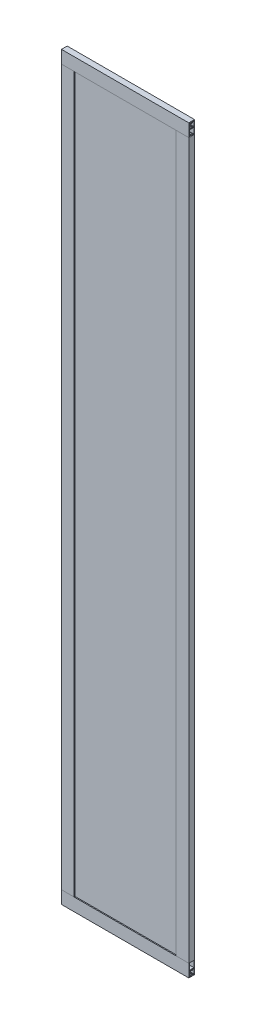
from build123d import *

# Parameters (mm, degrees)
MEMBER_1_DEPTH   = 398.5
MEMBER_1_2_DEPTH = 398.5
MEMBER_1_3_DEPTH = 2319
MEMBER_1_4_DEPTH = 2319
EXTRUDE_START    = -3.1
SKETCH_2_W       = 352.5
SKETCH_2_H       = 2271
EXTRUDE_1_DEPTH  = 10


with BuildPart() as part:
    # Sketch1 → Member 1 (new body)
    with BuildSketch(Plane(origin=(-199.25, 1158.5, 0), x_dir=(0, 0, -1), z_dir=(1, 0, 0))):
        Polygon((7, -38.5), (5.9, -38.5), (5.9, -40), (7, -40), (9, -40), (9, 0), (-9, 0), (-9, -40), (-7, -40), (-5.9, -40), (-5.9, -38.5), (-7, -38.5), (-7, -20), (7, -20), align=None)
        with BuildLine():
            Line((-1.341640786, -18), (1.341640786, -18))
            ThreePointArc((1.341640786, -18), (1.799302724, -16.749903013), (1.272792206, -15.527207794))
            ThreePointArc((1.272792206, -15.527207794), (1.272792206, -14.749390335), (2.050609665, -14.749390335))
            ThreePointArc((2.050609665, -14.749390335), (2.853462499, -16.282552641), (2.640075756, -18))
            Line((2.640075756, -18), (7, -18))
            Line((7, -18), (7, -3))
            Line((7, -3), (2.640075756, -3))
            ThreePointArc((2.640075756, -3), (2.853462499, -4.717447359), (2.050609665, -6.250609665))
            ThreePointArc((2.050609665, -6.250609665), (1.272792206, -6.250609665), (1.272792206, -5.472792206))
            ThreePointArc((1.272792206, -5.472792206), (1.799302724, -4.250096987), (1.341640786, -3))
            Line((1.341640786, -3), (-1.341640786, -3))
            ThreePointArc((-1.341640786, -3), (-1.799302724, -4.250096987), (-1.272792206, -5.472792206))
            ThreePointArc((-1.272792206, -5.472792206), (-1.272792206, -6.250609665), (-2.050609665, -6.250609665))
            ThreePointArc((-2.050609665, -6.250609665), (-2.853462499, -4.717447359), (-2.640075756, -3))
            Line((-2.640075756, -3), (-7, -3))
            Line((-7, -3), (-7, -18))
            Line((-7, -18), (-2.640075756, -18))
            ThreePointArc((-2.640075756, -18), (-2.853462499, -16.282552641), (-2.050609665, -14.749390335))
            ThreePointArc((-2.050609665, -14.749390335), (-1.272792206, -14.749390335), (-1.272792206, -15.527207794))
            ThreePointArc((-1.272792206, -15.527207794), (-1.799302724, -16.749903013), (-1.341640786, -18))
        make_face(mode=Mode.SUBTRACT)
    extrude(amount=MEMBER_1_DEPTH)


with BuildPart() as body_2:
    # Sketch1 on segment 2 (carried to segment 2) → Member 1 2 (new body)
    with BuildSketch(Plane(origin=(-199.25, -1158.5, 0), x_dir=(0, 0, 1), z_dir=(1, 0, 0))):
        Polygon((7, -38.5), (5.9, -38.5), (5.9, -40), (7, -40), (9, -40), (9, 0), (-9, 0), (-9, -40), (-7, -40), (-5.9, -40), (-5.9, -38.5), (-7, -38.5), (-7, -20), (7, -20), align=None)
        with BuildLine():
            Line((-1.341640786, -18), (1.341640786, -18))
            ThreePointArc((1.341640786, -18), (1.799302724, -16.749903013), (1.272792206, -15.527207794))
            ThreePointArc((1.272792206, -15.527207794), (1.272792206, -14.749390335), (2.050609665, -14.749390335))
            ThreePointArc((2.050609665, -14.749390335), (2.853462499, -16.282552641), (2.640075756, -18))
            Line((2.640075756, -18), (7, -18))
            Line((7, -18), (7, -3))
            Line((7, -3), (2.640075756, -3))
            ThreePointArc((2.640075756, -3), (2.853462499, -4.717447359), (2.050609665, -6.250609665))
            ThreePointArc((2.050609665, -6.250609665), (1.272792206, -6.250609665), (1.272792206, -5.472792206))
            ThreePointArc((1.272792206, -5.472792206), (1.799302724, -4.250096987), (1.341640786, -3))
            Line((1.341640786, -3), (-1.341640786, -3))
            ThreePointArc((-1.341640786, -3), (-1.799302724, -4.250096987), (-1.272792206, -5.472792206))
            ThreePointArc((-1.272792206, -5.472792206), (-1.272792206, -6.250609665), (-2.050609665, -6.250609665))
            ThreePointArc((-2.050609665, -6.250609665), (-2.853462499, -4.717447359), (-2.640075756, -3))
            Line((-2.640075756, -3), (-7, -3))
            Line((-7, -3), (-7, -18))
            Line((-7, -18), (-2.640075756, -18))
            ThreePointArc((-2.640075756, -18), (-2.853462499, -16.282552641), (-2.050609665, -14.749390335))
            ThreePointArc((-2.050609665, -14.749390335), (-1.272792206, -14.749390335), (-1.272792206, -15.527207794))
            ThreePointArc((-1.272792206, -15.527207794), (-1.799302724, -16.749903013), (-1.341640786, -18))
        make_face(mode=Mode.SUBTRACT)
    extrude(amount=MEMBER_1_2_DEPTH)


with BuildPart() as body_3:
    # Sketch1 on segment 3 (carried to segment 3) → Member 1 3 (new body)
    with BuildSketch(Plane(origin=(-199.25, 1159.5, 0), x_dir=(0, 0, 1), z_dir=(0, -1, 0))):
        Polygon((7, -38.5), (5.9, -38.5), (5.9, -40), (7, -40), (9, -40), (9, 0), (-9, 0), (-9, -40), (-7, -40), (-5.9, -40), (-5.9, -38.5), (-7, -38.5), (-7, -20), (7, -20), align=None)
        with BuildLine():
            Line((-1.341640786, -18), (1.341640786, -18))
            ThreePointArc((1.341640786, -18), (1.799302724, -16.749903013), (1.272792206, -15.527207794))
            ThreePointArc((1.272792206, -15.527207794), (1.272792206, -14.749390335), (2.050609665, -14.749390335))
            ThreePointArc((2.050609665, -14.749390335), (2.853462499, -16.282552641), (2.640075756, -18))
            Line((2.640075756, -18), (7, -18))
            Line((7, -18), (7, -3))
            Line((7, -3), (2.640075756, -3))
            ThreePointArc((2.640075756, -3), (2.853462499, -4.717447359), (2.050609665, -6.250609665))
            ThreePointArc((2.050609665, -6.250609665), (1.272792206, -6.250609665), (1.272792206, -5.472792206))
            ThreePointArc((1.272792206, -5.472792206), (1.799302724, -4.250096987), (1.341640786, -3))
            Line((1.341640786, -3), (-1.341640786, -3))
            ThreePointArc((-1.341640786, -3), (-1.799302724, -4.250096987), (-1.272792206, -5.472792206))
            ThreePointArc((-1.272792206, -5.472792206), (-1.272792206, -6.250609665), (-2.050609665, -6.250609665))
            ThreePointArc((-2.050609665, -6.250609665), (-2.853462499, -4.717447359), (-2.640075756, -3))
            Line((-2.640075756, -3), (-7, -3))
            Line((-7, -3), (-7, -18))
            Line((-7, -18), (-2.640075756, -18))
            ThreePointArc((-2.640075756, -18), (-2.853462499, -16.282552641), (-2.050609665, -14.749390335))
            ThreePointArc((-2.050609665, -14.749390335), (-1.272792206, -14.749390335), (-1.272792206, -15.527207794))
            ThreePointArc((-1.272792206, -15.527207794), (-1.799302724, -16.749903013), (-1.341640786, -18))
        make_face(mode=Mode.SUBTRACT)
    extrude(amount=MEMBER_1_3_DEPTH)

    # Member 1 3 end butt 1
    split(bisect_by=Plane(origin=(-199.25, 1118.5, 0), x_dir=(1, 0, 0), z_dir=(0, -1, 0)), keep=Keep.TOP)

    # Member 1 3 end butt 2
    split(bisect_by=Plane(origin=(-199.25, -1118.5, 0), x_dir=(-1, 0, 0), z_dir=(0, 1, 0)), keep=Keep.TOP)


with BuildPart() as body_4:
    # Sketch1 on segment 4 (carried to segment 4) → Member 1 4 (new body)
    with BuildSketch(Plane(origin=(199.25, 1159.5, 0), x_dir=(0, 0, -1), z_dir=(0, -1, 0))):
        Polygon((7, -38.5), (5.9, -38.5), (5.9, -40), (7, -40), (9, -40), (9, 0), (-9, 0), (-9, -40), (-7, -40), (-5.9, -40), (-5.9, -38.5), (-7, -38.5), (-7, -20), (7, -20), align=None)
        with BuildLine():
            Line((-1.341640786, -18), (1.341640786, -18))
            ThreePointArc((1.341640786, -18), (1.799302724, -16.749903013), (1.272792206, -15.527207794))
            ThreePointArc((1.272792206, -15.527207794), (1.272792206, -14.749390335), (2.050609665, -14.749390335))
            ThreePointArc((2.050609665, -14.749390335), (2.853462499, -16.282552641), (2.640075756, -18))
            Line((2.640075756, -18), (7, -18))
            Line((7, -18), (7, -3))
            Line((7, -3), (2.640075756, -3))
            ThreePointArc((2.640075756, -3), (2.853462499, -4.717447359), (2.050609665, -6.250609665))
            ThreePointArc((2.050609665, -6.250609665), (1.272792206, -6.250609665), (1.272792206, -5.472792206))
            ThreePointArc((1.272792206, -5.472792206), (1.799302724, -4.250096987), (1.341640786, -3))
            Line((1.341640786, -3), (-1.341640786, -3))
            ThreePointArc((-1.341640786, -3), (-1.799302724, -4.250096987), (-1.272792206, -5.472792206))
            ThreePointArc((-1.272792206, -5.472792206), (-1.272792206, -6.250609665), (-2.050609665, -6.250609665))
            ThreePointArc((-2.050609665, -6.250609665), (-2.853462499, -4.717447359), (-2.640075756, -3))
            Line((-2.640075756, -3), (-7, -3))
            Line((-7, -3), (-7, -18))
            Line((-7, -18), (-2.640075756, -18))
            ThreePointArc((-2.640075756, -18), (-2.853462499, -16.282552641), (-2.050609665, -14.749390335))
            ThreePointArc((-2.050609665, -14.749390335), (-1.272792206, -14.749390335), (-1.272792206, -15.527207794))
            ThreePointArc((-1.272792206, -15.527207794), (-1.799302724, -16.749903013), (-1.341640786, -18))
        make_face(mode=Mode.SUBTRACT)
    extrude(amount=MEMBER_1_4_DEPTH)

    # Member 1 4 end butt 1
    split(bisect_by=Plane(origin=(199.25, 1118.5, 0), x_dir=(1, 0, 0), z_dir=(0, -1, 0)), keep=Keep.TOP)

    # Member 1 4 end butt 2
    split(bisect_by=Plane(origin=(199.25, -1118.5, 0), x_dir=(-1, 0, 0), z_dir=(0, 1, 0)), keep=Keep.TOP)


with BuildPart() as body_5:
    # 草图2 → 凸台-拉伸1 (new body)
    with BuildSketch(Plane.XY.offset(9).offset(EXTRUDE_START)):
        Rectangle(SKETCH_2_W, SKETCH_2_H)
    extrude(amount=-EXTRUDE_1_DEPTH)


solid = Compound([part.part, body_2.part, body_3.part, body_4.part, body_5.part])
